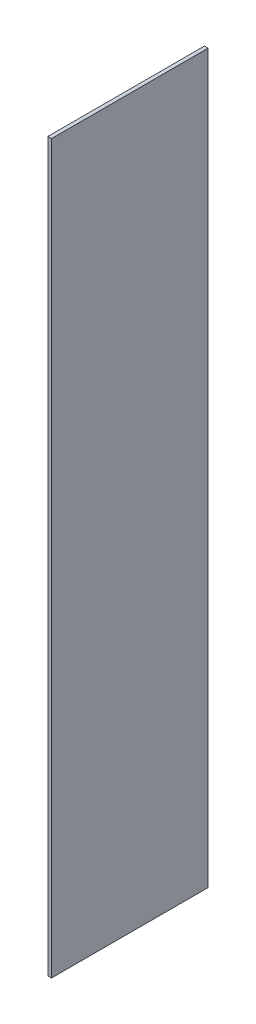
SolidWorks part; units mm, degrees
ref_plane "Front Plane" through (0, 0, 0) normal (0, 0, 1) x (1, 0, 0)
ref_plane "Top Plane" through (0, 0, 0) normal (0, 1, 0) x (1, 0, 0)
ref_plane "Right Plane" through (0, 0, 0) normal (1, 0, 0) x (0, 0, -1)
sketch "Sketch1" plane through (0, 0, 0) normal (0, 0, 1) x (1, 0, 0)
  line L1 (0.75, 148.5) -> (-0.75, 148.5)
  line L2 (0.75, 148.5) -> (0.75, -148.5)
  line L3 (0.75, -148.5) -> (-0.75, -148.5)
  line L4 (-0.75, 148.5) -> (-0.75, -148.5)
  line L5 (0.75, 148.5) -> (-0.75, -148.5) construction
  line L6 (0.75, -148.5) -> (-0.75, 148.5) construction
  point P0 (0, 0)
  dimension "D1" = 1.5
  dimension "D2" = 297
extrude "Boss-Extrude1" add sketch "Sketch1" along normal mid plane 64
